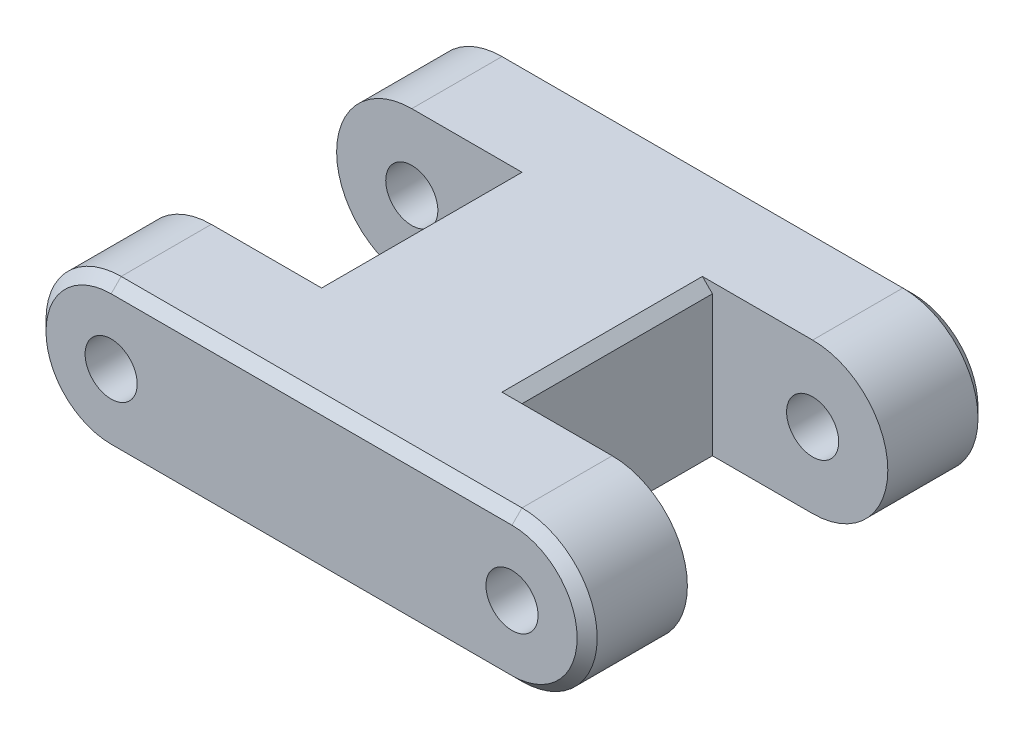
SolidWorks part; units mm, degrees
ref_plane "Front Plane" through (0, 0, 0) normal (0, 0, 1) x (1, 0, 0)
ref_plane "Top Plane" through (0, 0, 0) normal (0, 1, 0) x (1, 0, 0)
ref_plane "Right Plane" through (0, 0, 0) normal (1, 0, 0) x (0, 0, -1)
other "Configuration Table"
sketch "Sketch1" plane through (0, 0, 0) normal (0, 0, 1) x (1, 0, 0)
  line L0 (0, 0) -> (-40, 0) construction
  line L1 (0, -7.5) -> (-40, -7.5)
  line L2 (0, 7.5) -> (-40, 7.5)
  arc A0 (0, -7.5) -> (0, 7.5) centre (0, 0) ccw
  arc A1 (-40, 7.5) -> (-40, -7.5) centre (-40, 0) ccw
  circle A2 centre (0, 0) radius 2.6
  circle A3 centre (-40, 0) radius 2.6
  point P3 (-20, 0)
  dimension "D1" = 7.5
  dimension "D3" = 5.2
  dimension "D4" = 5.2
  dimension "D2" = 40
extrude "Boss-Extrude1" add sketch "Sketch1" along normal mid plane 10
sketch "Sketch2" plane through (0, 0, -5) normal (0, 0, -1) x (-1, 0, 0)
  line L0 (20, 7.5) -> (20, -7.5) construction
  line L1 (0, 7.5) -> (40, 7.5) construction
  line L2 (40, -7.5) -> (0, -7.5) construction
  line L3 (0, 0) -> (40, 0) construction
  line L5 (10, 7.5) -> (30, 7.5)
  line L6 (10, 7.5) -> (10, -7.5)
  line L7 (10, -7.5) -> (30, -7.5)
  line L8 (30, 7.5) -> (30, -7.5)
  line L9 (10, 7.5) -> (30, -7.5) construction
  line L10 (10, -7.5) -> (30, 7.5) construction
  point P10 (20, 0)
  dimension "D1" = 20
extrude "Boss-Extrude2" add sketch "Sketch2" along normal blind 20
sketch "Sketch3" plane through (0, 0, -25) normal (0, 0, -1) x (-1, 0, 0)
  line L0 (0, 0) -> (40, 0) construction
  line L1 (0, 7.5) -> (40, 7.5)
  line L2 (0, -7.5) -> (40, -7.5)
  arc A0 (0, 7.5) -> (0, -7.5) centre (0, 0) ccw
  arc A1 (40, -7.5) -> (40, 7.5) centre (40, 0) ccw
  circle A2 centre (0, 0) radius 2.6
  circle A3 centre (40, 0) radius 2.6
  point P4 (20, 0)
  dimension "D1" = 7.5
extrude "Boss-Extrude3" add sketch "Sketch3" along normal blind 10
chamfer "Chamfer1" distance 1 angle 45 10 edges at (-10, 7.5, -15) (-30, 7.5, -15) (-47.5, 0, -35) (-20, -7.5, -35) (-20, 7.5, -35) (7.5, 0, -35) (-47.5, 0, 5) (-20, -7.5, 5) (7.5, 0, 5) (-20, 7.5, 5)
